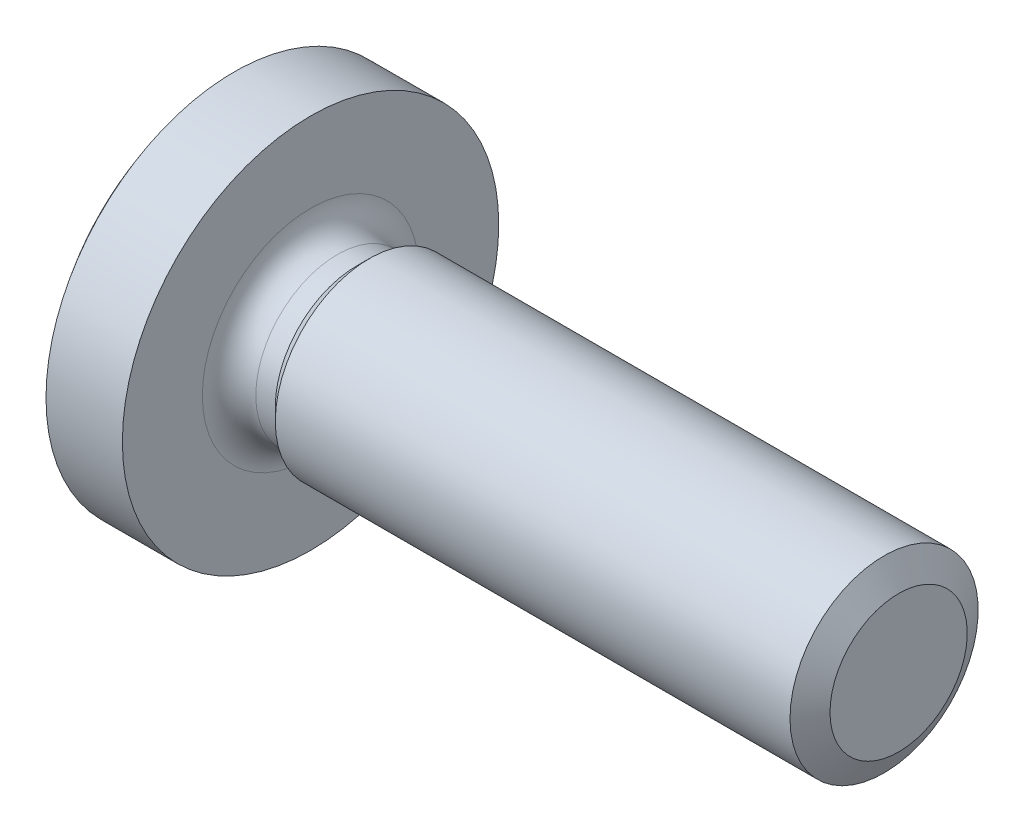
from build123d import *


with BuildPart() as part:
    # 草图2 → Revolve 709 (revolve)
    with BuildSketch(Plane.XY, mode=Mode.PRIVATE) as revolve_709_sk:
        with BuildLine():
            Line((0, 0), (31, 0))
            Line((31, 0), (31, 4))
            Line((31, 4), (8.5, 4))
            Line((8.5, 4), (7.964, 3.464))
            Line((7.964, 3.464), (7.136, 3.464))
            ThreePointArc((7.136, 3.464), (6.332726697, 3.796726697), (6, 4.6))
            Line((6, 4.6), (6, 8))
            Line((6, 8), (2.753049234, 8))
            ThreePointArc((2.753049234, 8), (0.707515305, 4.230226947), (0, 0))
        make_face()
    revolve(revolve_709_sk.sketch.rotate(Axis((-1.331757704, 0, 0), (1, 0, 0)), 90), axis=Axis((-1.331757704, 0, 0), (1, 0, 0)))

    # 草图3 → 切除-旋转1 (revolve, cut)
    with BuildSketch(Plane.XY, mode=Mode.PRIVATE) as cut_revolve_1_sk:
        Polygon((30.381770007, 4), (31.631770007, 4), (31, 2.9175), align=None)
    revolve(cut_revolve_1_sk.sketch.rotate(Axis((-0.242766179, 0, 0), (1, 0, 0)), 90), axis=Axis((-0.242766179, 0, 0), (1, 0, 0)), mode=Mode.SUBTRACT)

    # 草图5 → 切除-放样1 section 0
    with BuildSketch(Plane(origin=(0, 0, 0), x_dir=(0, 0, -1), z_dir=(1, 0, 0)), mode=Mode.PRIVATE) as loft_1_s0:
        with BuildLine():
            Line((0.625, 4.5), (-0.625, 4.5))
            Line((-0.625, 4.5), (-0.625, -4.5))
            Line((-0.625, -4.5), (0.625, -4.5))
            Line((0.625, -4.5), (0.625, 4.5))
        make_face()
    loft_1 = loft([Vertex(4.6, 0, 0), loft_1_s0.sketch], mode=Mode.SUBTRACT)

    # 镜向1: 切除-放样1 across plane
    add(loft_1.mirror(Plane(origin=(0, 0, 0), x_dir=(0, 0.7071067811865462, 0.7071067811865488), z_dir=(0, -0.7071067811865488, 0.7071067811865462))), mode=Mode.SUBTRACT)


solid = part.part
